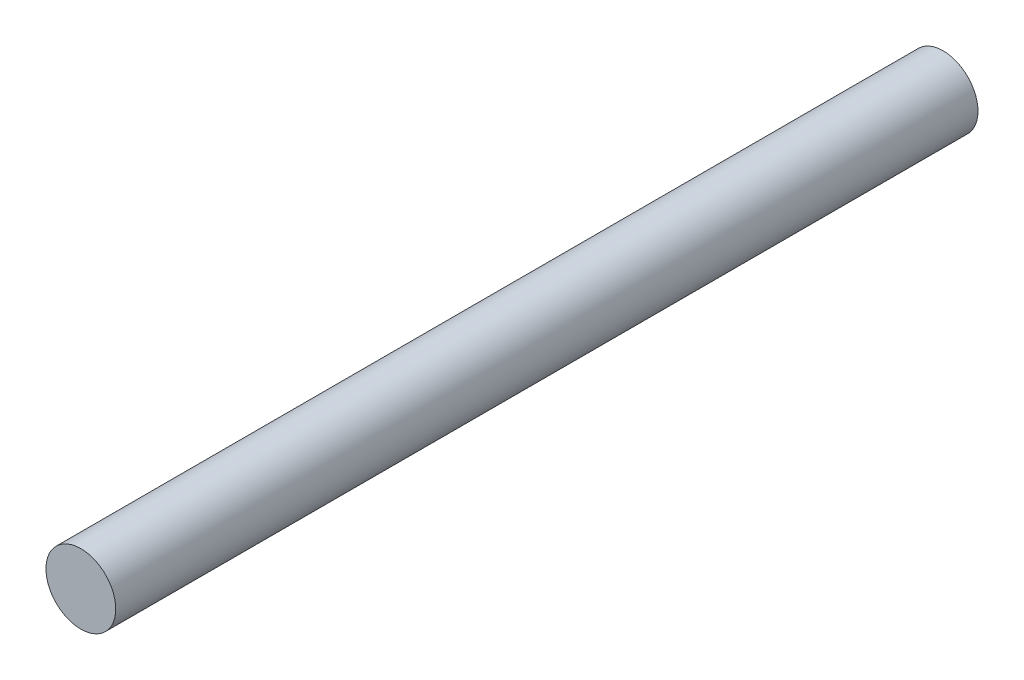
SolidWorks part; units mm, degrees
ref_plane "前视基准面" through (0, 0, 0) normal (0, 0, 1) x (1, 0, 0)
ref_plane "上视基准面" through (0, 0, 0) normal (0, 1, 0) x (1, 0, 0)
ref_plane "右视基准面" through (0, 0, 0) normal (1, 0, 0) x (0, 0, -1)
sketch "草图1" plane through (0, 0, 0) normal (0, 0, 1) x (1, 0, 0)
  circle A0 centre (0, 0) radius 8.5
  dimension "D1" = 17
extrude "凸台-拉伸1" add sketch "草图1" along normal blind 210
